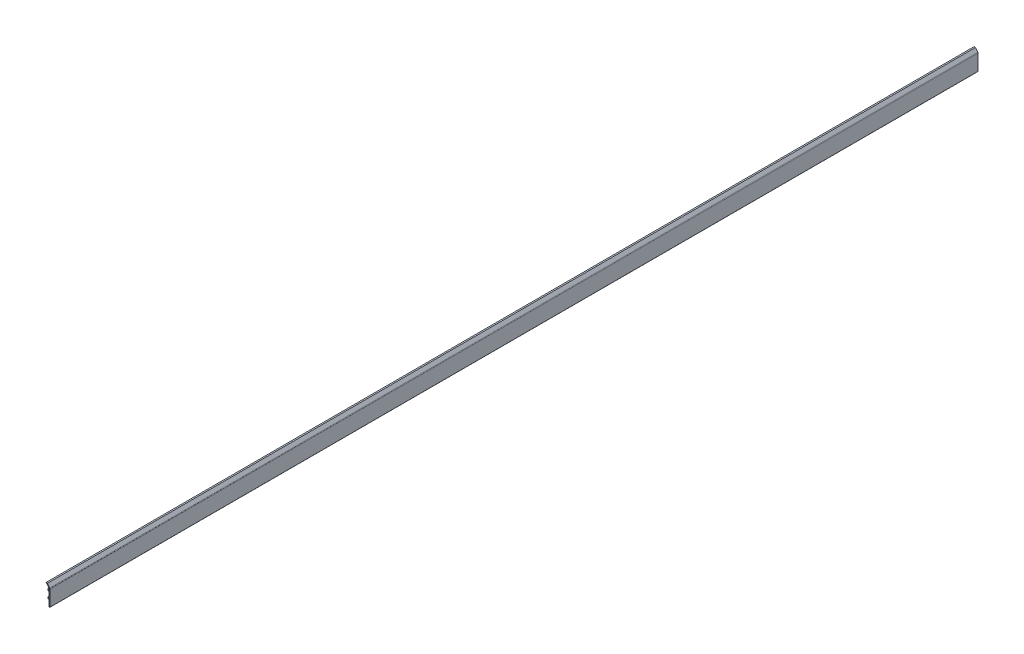
from build123d import *

# Parameters (mm, degrees)
EXTRUDE_1_DEPTH = 1108


with BuildPart() as part:
    # 草图2 → 凸台-拉伸1 (new, symmetric)
    with BuildSketch(Plane.XY):
        with BuildLine():
            Line((-2.699712502, 32.249908534), (-2.499724552, 32.249908534))
            ThreePointArc((-2.499724552, 32.249908534), (-2.075486045, 32.425633877), (-1.899760702, 32.849872384))
            Line((-1.899760702, 32.849872384), (-1.899760702, 36.12977276))
            ThreePointArc((-1.899760702, 36.12977276), (-1.864615633, 36.214620461), (-1.779767932, 36.24976553))
            Line((-1.779767932, 36.24976553), (0, 36.24976553))
            Line((0, 36.24976553), (0.000764104, 20.44942184))
            Line((0.000764104, 20.44942184), (-2.498960448, 20.44942184))
            ThreePointArc((-2.498960448, 20.44942184), (-2.781786119, 20.332271611), (-2.898936348, 20.04944594))
            Line((-2.898936348, 20.04944594), (-2.898936348, 15.649613044))
            ThreePointArc((-2.898936348, 15.649613044), (-2.840361233, 15.508200208), (-2.698948398, 15.449625094))
            Line((-2.698948398, 15.449625094), (-2.498960448, 15.449625094))
            ThreePointArc((-2.498960448, 15.449625094), (-2.074721941, 15.625350437), (-1.898996598, 16.049588944))
            Line((-1.898996598, 16.049588944), (-1.898996598, 19.32948932))
            ThreePointArc((-1.898996598, 19.32948932), (-1.863851529, 19.414337021), (-1.779003828, 19.44948209))
            Line((-1.779003828, 19.44948209), (0.000764104, 19.44948209))
            Line((0.000764104, 19.44948209), (0, 0))
            Line((0, 0), (1.5, 0))
            ThreePointArc((1.5, 0), (1.853553391, 0.146446609), (2, 0.5))
            Line((2, 0.5), (2, 38.058011928))
            ThreePointArc((2, 38.058011928), (1.844147591, 39.012383177), (1.392783679, 39.867593721))
            Line((1.392783679, 39.867593721), (-4, 46.998393128))
            Line((-4, 46.998393128), (-7.4, 46.998393128))
            Line((-7.4, 46.998393128), (-7.4, 45.998393128))
            Line((-7.4, 45.998393128), (-5.751273316, 45.998393128))
            Line((-5.751273316, 45.998393128), (-0.607216321, 39.196481397))
            ThreePointArc((-0.607216321, 39.196481397), (-0.155852409, 38.341270854), (0, 37.386899605))
            Line((0, 37.386899605), (0, 37.24970528))
            Line((0, 37.24970528), (-2.499724552, 37.24970528))
            ThreePointArc((-2.499724552, 37.24970528), (-2.782550223, 37.132555051), (-2.899700452, 36.84972938))
            Line((-2.899700452, 36.84972938), (-2.899700452, 32.449896484))
            ThreePointArc((-2.899700452, 32.449896484), (-2.841125337, 32.308483648), (-2.699712502, 32.249908534))
        make_face()
    extrude(amount=EXTRUDE_1_DEPTH, both=True)


solid = part.part
